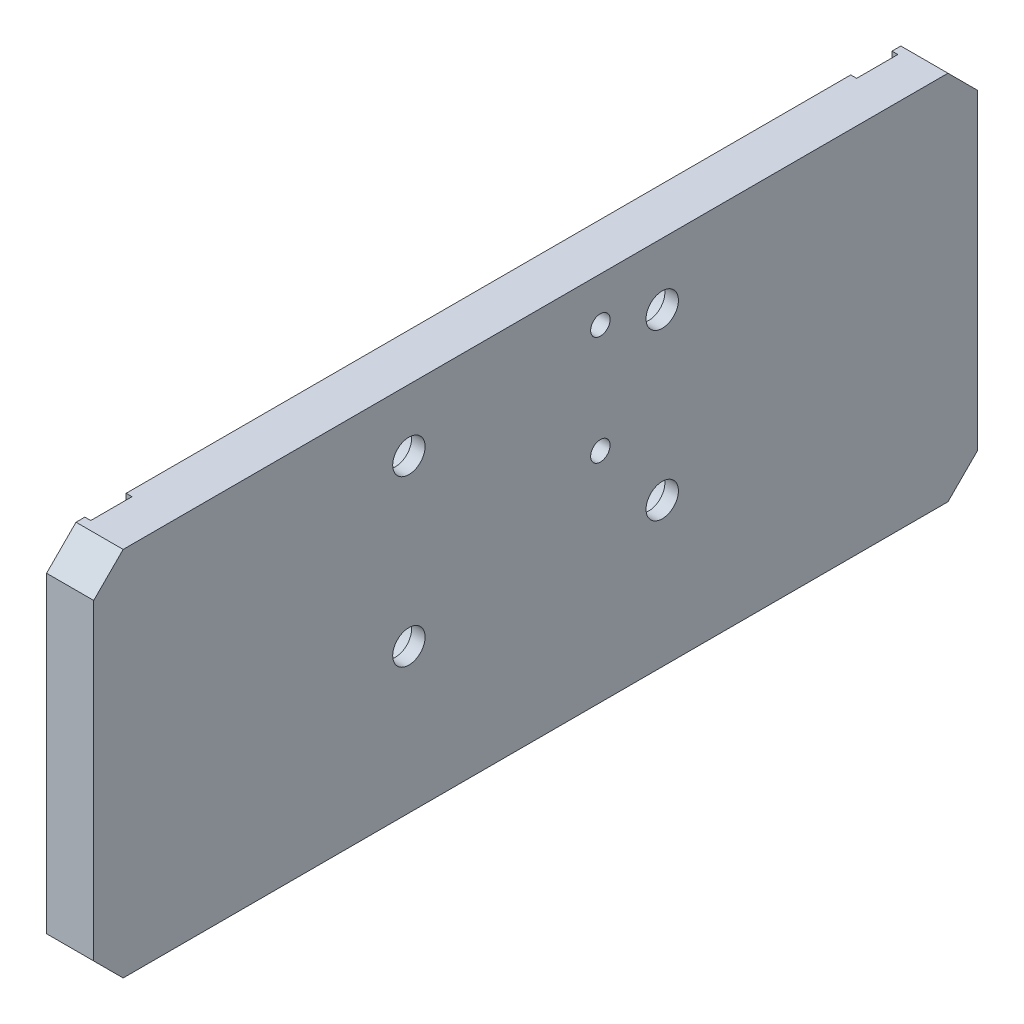
SolidWorks part; units mm, degrees
material "AL6061"
ref_plane "Front Plane" through (0, 0, 0) normal (0, 0, 1) x (1, 0, 0)
ref_plane "Top Plane" through (0, 0, 0) normal (0, 1, 0) x (1, 0, 0)
ref_plane "Right Plane" through (0, 0, 0) normal (1, 0, 0) x (0, 0, -1)
sketch "Sketch1" plane through (0, 0, 0) normal (1, 0, 0) x (0, 0, -1)
  line L1 (-75, -31.5) -> (75, -31.5)
  line L2 (-75, -31.5) -> (-75, 31.5)
  line L3 (-75, 31.5) -> (75, 31.5)
  line L4 (75, -31.5) -> (75, 31.5)
  line L5 (-75, -31.5) -> (75, 31.5) construction
  line L6 (-75, 31.5) -> (75, -31.5) construction
  point P0 (0, 0)
  dimension "D1" = 150
  dimension "D2" = 63
extrude "Boss-Extrude1" add sketch "Sketch1" along normal blind 8
hole_wizard "M4 Tapped Hole1" positions "Sketch10" profile "Sketch11" tap size "M4" standard "GB"
sketch "Sketch10" plane through (0, 0, 0) normal (-1, 0, 0) x (0, 0, 1)
  point P0 (-11, 24)
  point P3 (-11, 5.5)
sketch "Sketch11" plane through (0, 24, -11) normal (0, 1, 0) x (0, 0, 1)
  line L0 (0, 0) -> (0, 11.0914)
  line L1 (0, 11.0914) -> (1.65, 10.1)
  line L2 (1.65, 10.1) -> (1.65, 0)
  line L5 (1.65, 0) -> (0, 0)
  line L10 (0, 11.0914) -> (-1.65, 10.1) construction
  line L11 (0, -6.35) -> (0, 107.95) construction
  dimension "螺纹孔钻头直径" = 3.3
  dimension "螺纹孔钻头深度" = 10.1
  dimension "导头角度" = 118
cosmetic thread "Cosmetic Thread 13" parameters "D1"=8, "D2"=4
cosmetic thread "Cosmetic Thread 14" parameters "D1"=8, "D2"=4
hole_wizard "CBORE for M5 Hexagon socket head cap screws1" positions "Sketch14" profile "Sketch15" counterbore size "M5" standard "GB"
sketch "Sketch14" plane through (0, 0, 0) normal (-1, 0, 0) x (0, 0, 1)
  point P0 (21.5, 21)
  point P3 (21.5, -7)
  point P6 (-21.5, 21)
  point P9 (-21.5, -7)
sketch "Sketch15" plane through (0, 21, 21.5) normal (0, 1, 0) x (0, 0, 1)
  line L0 (0, 0) -> (0, 14.0524)
  line L1 (0, 14.0524) -> (2.75, 12.4)
  line L2 (2.75, 12.4) -> (2.75, 5.7)
  line L3 (2.75, 5.7) -> (5, 5.7)
  line L5 (5, 5.7) -> (5, 0.025)
  line L6 (5, 0.025) -> (5.025, 0)
  line L7 (5.025, 0) -> (0, 0)
  line L8 (-5, 0.025) -> (-5.025, 0) construction
  line L10 (0, 14.0524) -> (-2.75, 12.4) construction
  line L11 (0, -6.35) -> (0, 107.95) construction
  dimension "孔直径" = 5.5
  dimension "孔深度" = 12.4
  dimension "锥形沉头孔直径" = 10
  dimension "锥形沉头孔深度" = 5.7
  dimension "近端锥形沉头孔直径" = 10.05
  dimension "近端锥形沉头孔角度" = 90
  dimension "导头角度" = 118
hole_wizard "M2 Tapped Hole1" positions "Sketch8" profile "Sketch9" tap size "M2" standard "GB"
sketch "Sketch8" plane through (0, 0, 0) normal (-1, 0, 0) x (0, 0, 1)
  point P1 (-65, 18.5)
  point P4 (-65, 3.5)
  point P7 (-65, -11.5)
  point P10 (65, -11.5)
  point P13 (65, 3.5)
  point P16 (65, 18.5)
sketch "Sketch9" plane through (0, 18.5, -65) normal (0, 1, 0) x (0, 0, 1)
  line L0 (0, 0) -> (0, 6.6807)
  line L1 (0, 6.6807) -> (0.8, 6.2)
  line L2 (0.8, 6.2) -> (0.8, 0)
  line L5 (0.8, 0) -> (0, 0)
  line L10 (0, 6.6807) -> (-0.8, 6.2) construction
  line L11 (0, -6.35) -> (0, 107.95) construction
  dimension "螺纹孔钻头直径" = 1.6
  dimension "螺纹孔钻头深度" = 6.2
  dimension "导头角度" = 118
cosmetic thread "Cosmetic Thread 7" parameters "D1"=5, "D2"=2
cosmetic thread "Cosmetic Thread 8" parameters "D1"=5, "D2"=2
cosmetic thread "Cosmetic Thread 9" parameters "D1"=5, "D2"=2
cosmetic thread "Cosmetic Thread 10" parameters "D1"=5, "D2"=2
cosmetic thread "Cosmetic Thread 11" parameters "D1"=5, "D2"=2
cosmetic thread "Cosmetic Thread 12" parameters "D1"=5, "D2"=2
sketch "Sketch17" plane through (0, 0, 0) normal (-1, 0, 0) x (0, 0, 1)
  line L0 (65, 18.5) -> (65, -11.5) construction
  line L1 (-75, 31.5) -> (75, 31.5) construction
  line L2 (61.5, -31.5) -> (68.5, -31.5)
  line L3 (61.5, -31.5) -> (61.5, 31.5)
  line L4 (61.5, 31.5) -> (68.5, 31.5)
  line L5 (68.5, -31.5) -> (68.5, 31.5)
  line L6 (61.5, -31.5) -> (68.5, 31.5) construction
  line L7 (61.5, 31.5) -> (68.5, -31.5) construction
  line L8 (75, -31.5) -> (-75, -31.5) construction
  line L9 (0, 0) -> (0, 37.2668) construction
  line L10 (-61.5, 31.5) -> (-68.5, -31.5) construction
  line L11 (-61.5, -31.5) -> (-68.5, 31.5) construction
  line L12 (-65, 18.5) -> (-65, -11.5) construction
  line L13 (-68.5, -31.5) -> (-68.5, 31.5)
  line L14 (-61.5, 31.5) -> (-68.5, 31.5)
  line L15 (-61.5, -31.5) -> (-61.5, 31.5)
  line L16 (-61.5, -31.5) -> (-68.5, -31.5)
  point P4 (65, 0)
  point P22 (-65, 0)
  dimension "D1" = 7
extrude "Cut-Extrude1" cut sketch "Sketch17" against normal blind 1
chamfer "Chamfer1" distance 5 angle 45 4 edges at (4, 31.5, -75) (4, -31.5, -75) (4, 31.5, 75) (4, -31.5, 75)
